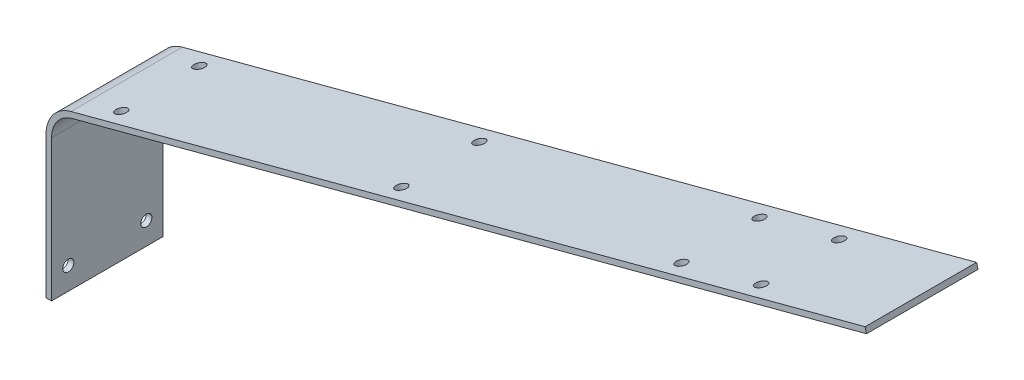
from build123d import *

# Parameters (mm, degrees)
EXTRUDE_THIN1_DEPTH  = 100
SKETCH2_R            = 5
CUT_EXTRUDE1_DEPTH   = 10
LPATTERN1_COUNT      = 2
LPATTERN1_PITCH      = 70
SKETCH3_R            = 5
CUT_EXTRUDE2_DEPTH   = 10
LPATTERN2_COUNT      = 3
LPATTERN2_PITCH      = 260
LPATTERN2_COUNT_DIR2 = 2
LPATTERN2_PITCH_DIR2 = 70
SKETCH4_R            = 5
CUT_EXTRUDE3_DEPTH   = 10
LPATTERN3_COUNT      = 2
LPATTERN3_PITCH      = 70


with BuildPart() as part:
    # Sketch1 → Extrude-Thin1 (new body)
    with BuildSketch(Plane.XY):
        with BuildLine():
            Line((0, 0), (0, 126.921326068))
            ThreePointArc((0, 126.921326068), (6.221950993, 145.213520727), (22.306959029, 155.918172804))
            Line((22.306959029, 155.918172804), (735, 345))
            Line((735, 345), (736.282173495, 340.167192211))
            Line((736.282173495, 340.167192211), (23.589132524, 151.085365014))
            ThreePointArc((23.589132524, 151.085365014), (10.184959161, 142.164821617), (5, 126.921326068))
            Line((5, 126.921326068), (5, 0))
            Line((5, 0), (0, 0))
        make_face()
    extrude(amount=EXTRUDE_THIN1_DEPTH)

    # Sketch2 → Cut-Extrude1 (cut)
    with BuildSketch(Plane(origin=(-37.178988327, 140.13618677, 0), x_dir=(0.9665615578617778, 0.25643469902455335, 0), z_dir=(-0.25643469902455335, 0.9665615578617778, 0))):
        with Locations(Location((686.892716192, -15, 0), (0, 0, 180))):
            Circle(SKETCH2_R)
    cut_extrude1 = extrude(amount=-CUT_EXTRUDE1_DEPTH, mode=Mode.SUBTRACT)

    # LPattern1: Cut-Extrude1 ×2
    with Locations(*[(0, 0, i * LPATTERN1_PITCH) for i in range(1, LPATTERN1_COUNT)]):
        add(cut_extrude1, mode=Mode.SUBTRACT)

    # Sketch3 → Cut-Extrude2 (cut)
    with BuildSketch(Plane(origin=(-37.178988327, 140.13618677, 0), x_dir=(0.9665615578617778, 0.25643469902455335, 0), z_dir=(-0.25643469902455335, 0.9665615578617778, 0))):
        with Locations(Location((612.892716192, -15, 0), (0, 0, 180))):
            Circle(SKETCH3_R)
    cut_extrude2 = extrude(amount=-CUT_EXTRUDE2_DEPTH, mode=Mode.SUBTRACT)

    # LPattern2: Cut-Extrude2 3 × 2
    with Locations(*[Vector(-0.9665615578617778, -0.25643469902455335, 0) * (i * LPATTERN2_PITCH) + Vector(0, 0, 1) * (j * LPATTERN2_PITCH_DIR2) for i in range(LPATTERN2_COUNT) for j in range(LPATTERN2_COUNT_DIR2) if (i, j) != (0, 0)]):
        add(cut_extrude2, mode=Mode.SUBTRACT)

    # Sketch4 → Cut-Extrude3 (cut)
    with BuildSketch(Plane.ZY):
        with Locations((85, 20)):
            Circle(SKETCH4_R)
    cut_extrude3 = extrude(amount=-CUT_EXTRUDE3_DEPTH, mode=Mode.SUBTRACT)

    # LPattern3: Cut-Extrude3 ×2
    with Locations(*[(0, 0, -i * LPATTERN3_PITCH) for i in range(1, LPATTERN3_COUNT)]):
        add(cut_extrude3, mode=Mode.SUBTRACT)


solid = part.part
